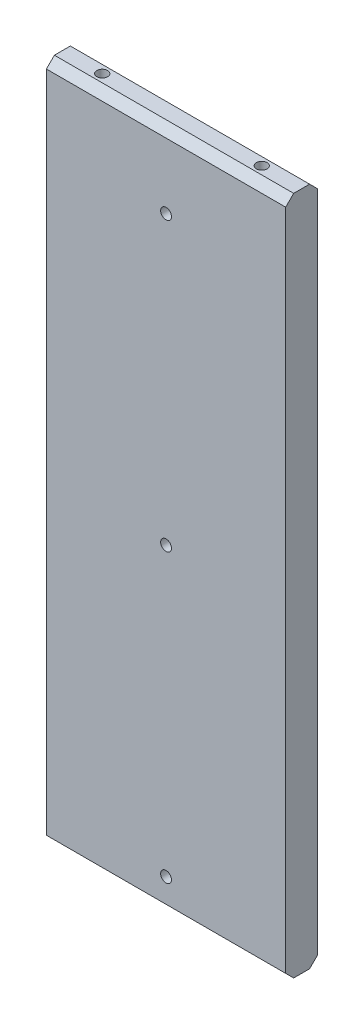
SolidWorks part; units mm, degrees
material "Q235"
ref_plane "Front Plane" through (0, 0, 0) normal (0, 0, 1) x (1, 0, 0)
ref_plane "Top Plane" through (0, 0, 0) normal (0, 1, 0) x (1, 0, 0)
ref_plane "Right Plane" through (0, 0, 0) normal (1, 0, 0) x (0, 0, -1)
sketch "Sketch1" plane through (0, 0, 0) normal (0, 0, 1) x (1, 0, 0)
  line L1 (0, 0) -> (150, 0)
  line L2 (0, 0) -> (0, 426)
  line L3 (0, 426) -> (150, 426)
  line L4 (150, 0) -> (150, 426)
  dimension "D1" = 426
  dimension "D2" = 150
extrude "Boss-Extrude1" add sketch "Sketch1" along normal blind 20
sketch "Sketch2" plane through (0, 0, 0) normal (0, 0, -1) x (-1, 0, 0)
  line L0 (0, 0) -> (-150, 0) construction
  line L1 (-85, 400) -> (-65, 400)
  line L2 (-85, 400) -> (-85, 0)
  line L3 (-85, 0) -> (-65, 0)
  line L4 (-65, 400) -> (-65, 0)
  line L5 (-75, 426) -> (-75, 400) construction
  line L6 (-150, 426) -> (0, 426) construction
  dimension "D1" = 20
  dimension "D2" = 26
extrude "Cut-Extrude1" cut sketch "Sketch2" against normal blind 3
hole_wizard "M8 Tapped Hole2" positions "Sketch3" profile "Sketch4" tap size "M8" standard "GB"
sketch "Sketch3" plane through (0, 0, 3) normal (0, 0, -1) x (-1, 0, 0)
  line L0 (-85, 0) -> (-65, 0) construction
  line L1 (-75, 0) -> (-75, 20) construction
  point P0 (-75, 20)
  point P2 (-75, 200)
  point P4 (-75, 380)
  dimension "D1" = 20
  dimension "D2" = 180
  dimension "D3" = 180
sketch "Sketch4" plane through (75, 20, 3) normal (1, 0, 0) x (0, 1, 0)
  line L0 (0, 0) -> (0, 21.7929)
  line L1 (0, 21.7929) -> (3.4, 19.75)
  line L2 (3.4, 19.75) -> (3.4, 0)
  line L5 (3.4, 0) -> (0, 0)
  line L10 (0, 21.7929) -> (-3.4, 19.75) construction
  line L11 (0, -6.35) -> (0, 107.95) construction
  dimension "螺纹孔钻头直径" = 6.8
  dimension "螺纹孔钻头深度" = 19.75
  dimension "导头角度" = 118
cosmetic thread "Cosmetic Thread1" parameters "D1"=16, "D2"=8
cosmetic thread "Cosmetic Thread2" parameters "D1"=16, "D2"=8
cosmetic thread "Cosmetic Thread3" parameters "D1"=16, "D2"=8
hole_wizard "M8 Tapped Hole1" positions "Sketch7" profile "Sketch8" tap size "M8" standard "GB"
sketch "Sketch7" plane through (0, 426, 0) normal (0, 1, 0) x (1, 0, 0)
  line L0 (75, -3) -> (75, -20) construction
  line L1 (65, -3) -> (85, -3) construction
  line L2 (150, -20) -> (0, -20) construction
  line L4 (0, -10) -> (25, -10) construction
  line L5 (0, -20) -> (0, 0) construction
  point P0 (25, -10)
  point P2 (125, -10)
  dimension "D1" = 100
cosmetic thread "Cosmetic Thread4" parameters "D1"=16, "D2"=8
cosmetic thread "Cosmetic Thread5" parameters "D1"=16, "D2"=8
sketch "Sketch8" plane through (25, 426, 10) normal (1, 0, 0) x (0, 0, 1)
  line L0 (0, 0) -> (0, 22.0429)
  line L1 (0, 22.0429) -> (3.4, 20)
  line L2 (3.4, 20) -> (3.4, 0)
  line L5 (3.4, 0) -> (0, 0)
  line L10 (0, 22.0429) -> (-3.4, 20) construction
  line L11 (0, -6.35) -> (0, 107.95) construction
  dimension "螺纹孔钻头直径" = 6.8
  dimension "螺纹孔钻头深度" = 20
  dimension "导头角度" = 118
chamfer "Chamfer1" distance 5 angle 45 2 edges at (75, 0, 20) (32.5, 0, 0)
chamfer "Chamfer2" distance 5 angle 45 2 edges at (75, 426, 20) (75, 426, 0)
